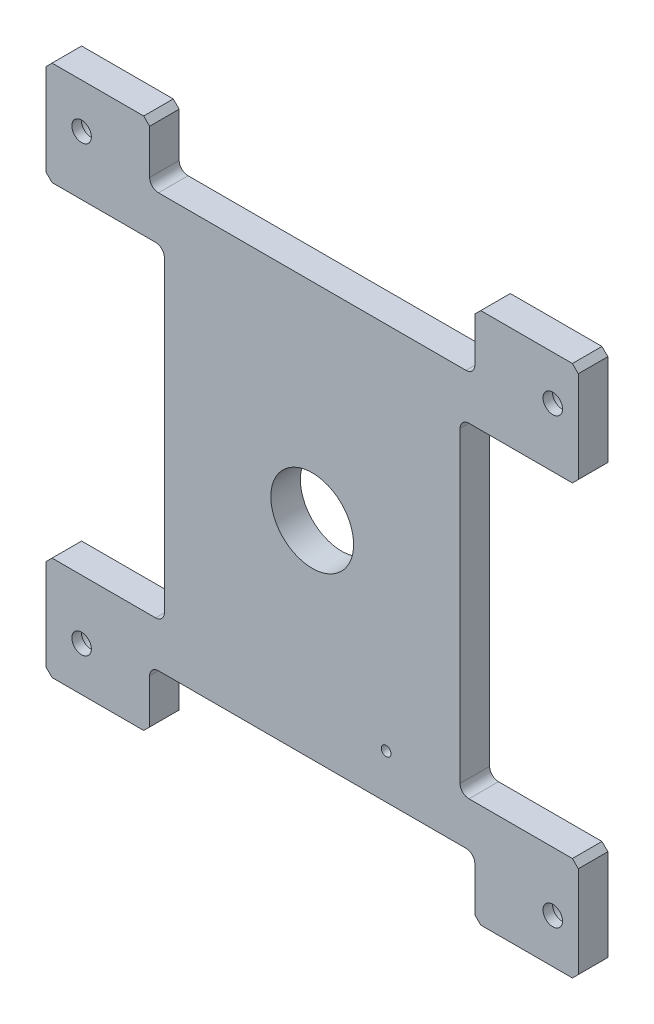
from build123d import *

# Parameters (mm, degrees)
BOSS_EXTRUDE1_DEPTH                                  = 10
SKETCH2_R                                            = 14
CUT_EXTRUDE1_DEPTH                                   = 128.671453348
M4_TAPPED_HOLE1_D                                    = 3.3
CBORE_FOR_M6_HEXAGON_SOCKET_HEAD_CAP_SCR_D           = 6.6
CBORE_FOR_M6_HEXAGON_SOCKET_HEAD_CAP_SCR_CBORE_D     = 11
CBORE_FOR_M6_HEXAGON_SOCKET_HEAD_CAP_SCR_CBORE_DEPTH = 6.8
CHAMFER1_SIZE                                        = 2
FILLET1_R                                            = 3


with BuildPart() as part:
    # Sketch1 → Boss-Extrude1 (new body)
    with BuildSketch(Plane.XY):
        Polygon((-90, 55), (-50, 55), (-50, -55), (-90, -55), (-90, -90), (-55, -90), (-55, -70), (55, -70), (55, -90), (90, -90), (90, -55), (50, -55), (50, 55), (90, 55), (90, 90), (55, 90), (55, 70), (-55, 70), (-55, 90), (-90, 90), align=None)
    extrude(amount=BOSS_EXTRUDE1_DEPTH)

    # Sketch2 → Cut-Extrude1 (cut, through all)
    with BuildSketch(Plane(origin=(0, 0, 0), x_dir=(-1, 0, 0), z_dir=(0, 0, -1))):
        Circle(SKETCH2_R)
    extrude(amount=-CUT_EXTRUDE1_DEPTH, mode=Mode.SUBTRACT)

    # M4 Tapped Hole1 (through all)
    with Locations(Plane.XY.offset(10)):
        with Locations((25, -55)):
            Hole(M4_TAPPED_HOLE1_D / 2)

    # CBORE for M6 Hexagon socket head cap screws1 (through all)
    with Locations(Plane(origin=(0, 0, 0), x_dir=(-1, 0, 0), z_dir=(0, 0, -1))):
        with Locations((78, -75), (78, 75), (-81.36030205, 75), (-81.36030205, -75)):
            CounterBoreHole(CBORE_FOR_M6_HEXAGON_SOCKET_HEAD_CAP_SCR_D / 2, CBORE_FOR_M6_HEXAGON_SOCKET_HEAD_CAP_SCR_CBORE_D / 2, CBORE_FOR_M6_HEXAGON_SOCKET_HEAD_CAP_SCR_CBORE_DEPTH)

    # Chamfer1
    chamfer1_edges = [part.edges().sort_by_distance(p)[0] for p in [
        (-90, 55, 5),
        (-90, 90, 5),
        (-55, 90, 5),
        (55, 90, 5),
        (90, 90, 5),
        (90, 55, 5),
        (90, -55, 5),
        (90, -90, 5),
        (55, -90, 5),
        (-55, -90, 5),
        (-90, -90, 5),
        (-90, -55, 5),
    ]]
    chamfer(chamfer1_edges, length=CHAMFER1_SIZE)

    # Fillet1
    fillet1_edges = [part.edges().sort_by_distance(p)[0] for p in [
        (-55, 70, 5),
        (55, 70, 5),
        (50, 55, 5),
        (50, -55, 5),
        (55, -70, 5),
        (-55, -70, 5),
        (-50, -55, 5),
        (-50, 55, 5),
    ]]
    fillet(fillet1_edges, radius=FILLET1_R)


solid = part.part
